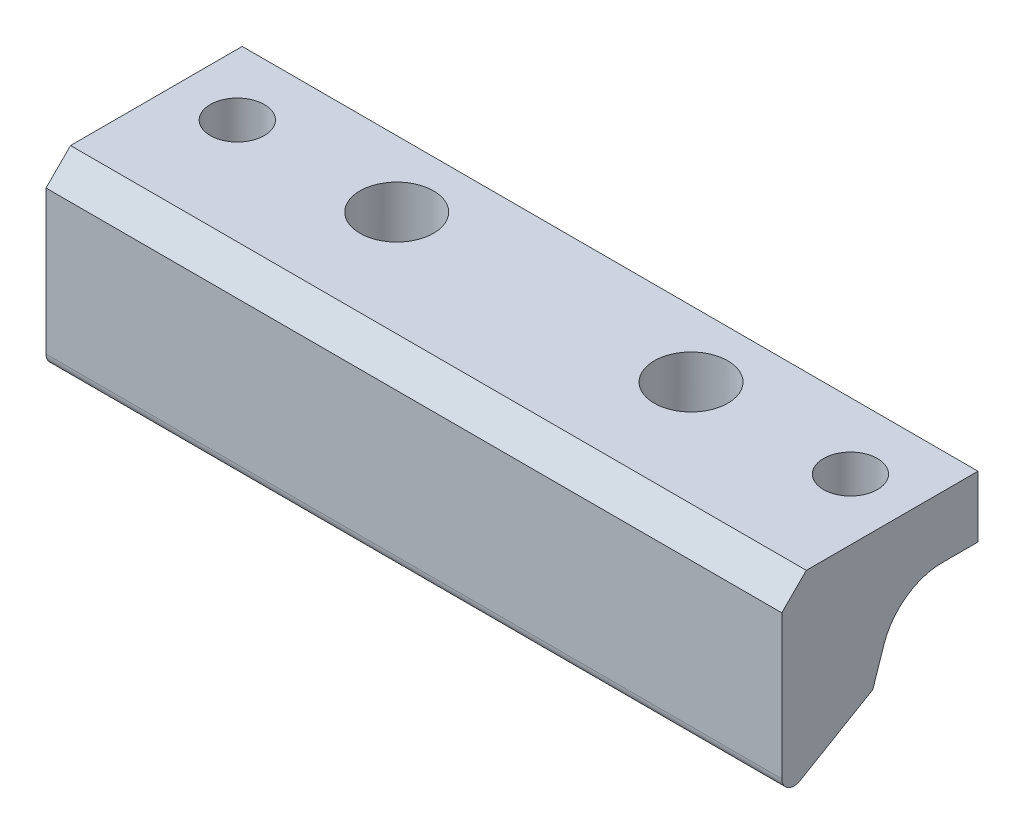
from build123d import *

# Parameters (mm, degrees)
EXTRUDE_1_DEPTH     = 30
MM_1_D              = 3
CUT_EXTRUDE_1_DEPTH = 3.5
CUT_EXTRUDE_2_REACH = 19.682
SKETCH_15_R         = 1.1
CUT_EXTRUDE_3_DEPTH = 5


with BuildPart() as part:
    # 草图2 → 凸台-拉伸1 (new body)
    with BuildSketch(Plane(origin=(15, 0, 0), x_dir=(0, 0, -1), z_dir=(1, 0, 0))):
        with BuildLine():
            Line((0, -3.5), (1, -2.5))
            Line((1, -2.5), (8, -2.5))
            Line((8, -2.5), (8, -5))
            Line((8, -5), (6.535231383, -5))
            ThreePointArc((6.535231383, -5), (5.073455672, -5.471894537), (4.163523138, -6.709430585))
            Line((4.163523138, -6.709430585), (3.710344828, -8.068965517))
            Line((3.710344828, -8.068965517), (0.751935513, -9.794704284))
            ThreePointArc((0.751935513, -9.794704284), (0.250969637, -9.79638591), (0, -9.362814834))
            Line((0, -9.362814834), (0, -3.5))
        make_face()
    extrude(amount=-EXTRUDE_1_DEPTH)

    # 大小mm 暗销孔1 (through all)
    with Locations(Plane(origin=(0, -2.5, 0), x_dir=(1, 0, 0), z_dir=(0, 1, 0))):
        with Locations((6, 5.3), (-6, 5.3)):
            Hole(MM_1_D / 2)

    # 草图13 → 切除-拉伸1 (cut)
    with BuildSketch(Plane(origin=(0, -8.5, 0), x_dir=(1, 0, 0), z_dir=(0, 1, 0))):
        with BuildLine():
            ThreePointArc((10.927039915, 6.535231383), (12.5, 3.3), (14.072960085, 6.535231383))
            ThreePointArc((14.072960085, 6.535231383), (12.5, 7.186772784), (10.927039915, 6.535231383))
        make_face()
    extrude(amount=CUT_EXTRUDE_1_DEPTH, mode=Mode.SUBTRACT)

    # 草图14 → 切除-拉伸2 (cut, up to next)
    with BuildSketch(Plane.XZ.offset(5), mode=Mode.PRIVATE) as cut_extrude_2_sk1:
        with BuildLine():
            ThreePointArc((-10.927039915, -6.535231383), (-12.5, -3.3), (-14.072960085, -6.535231383))
            ThreePointArc((-14.072960085, -6.535231383), (-12.5, -7.186772784), (-10.927039915, -6.535231383))
        make_face()
    cut_extrude_2_tool1 = extrude(cut_extrude_2_sk1.sketch, amount=CUT_EXTRUDE_2_REACH, mode=Mode.PRIVATE) & part.part
    add(cut_extrude_2_tool1.solids().sort_by_distance((-12.5, -5, -5.261226))[0], mode=Mode.SUBTRACT)

    # 草图15 → 切除-拉伸3 (cut)
    with BuildSketch(Plane.XZ.offset(5)):
        with Locations(Location((12.5, -5.3, 0), (0, 0, 270))):
            Circle(SKETCH_15_R)
        with Locations(Location((-12.5, -5.3, 0), (0, 0, 270))):
            Circle(SKETCH_15_R)
    extrude(amount=-CUT_EXTRUDE_3_DEPTH, mode=Mode.SUBTRACT)


solid = part.part
